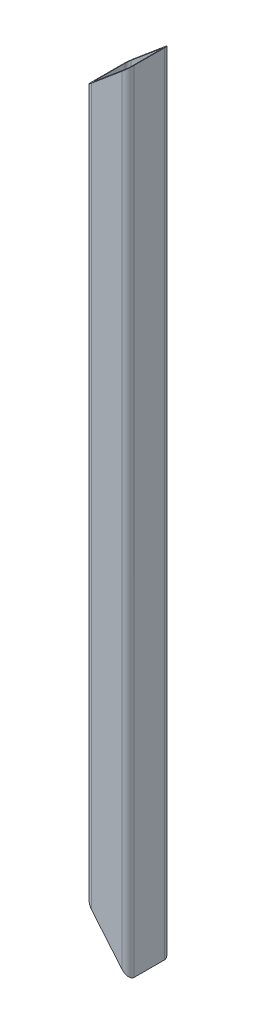
SolidWorks part; units mm, degrees
material "Q235B"
ref_plane "Front Plane" through (0, 0, 0) normal (0, 0, 1) x (1, 0, 0)
ref_plane "Top Plane" through (0, 0, 0) normal (0, 1, 0) x (1, 0, 0)
ref_plane "Right Plane" through (0, 0, 0) normal (1, 0, 0) x (0, 0, -1)
sketch "feature 17 (ProfileFeature) (+16 more in 12 files) Sketch1" plane through (0, 0, 0) normal (0, 0, 1) x (1, 0, 0)
  line L0 (0, 0) -> (0, 1302)
  dimension "D1" = 1302
other "feature 19 (WeldMemberFeat) (+4 more in 5 files) Cold-formed Hollow Structural Square Steel(gb t6728-2002) 70×70×5(1)"
ref_plane "Plane1" through (0, 0, 0) normal (0, 1, 0) x (-1, 0, 0)
sketch "Sketch1" plane through (0, 0, 0) normal (0, 1, 0) x (-1, 0, 0)
  line L0 (-25, -30) -> (25, -30)
  line L1 (-30, -25) -> (-30, 25)
  line L2 (25, 30) -> (-25, 30)
  line L3 (30, 25) -> (30, -25)
  line L4 (-25, -35) -> (25, -35)
  line L5 (-35, -25) -> (-35, 25)
  line L6 (25, 35) -> (-25, 35)
  line L7 (35, 25) -> (35, -25)
  arc A0 (35, 25) -> (25, 35) centre (25, 25) ccw
  arc A1 (25, -35) -> (35, -25) centre (25, -25) ccw
  arc A2 (-35, -25) -> (-25, -35) centre (-25, -25) ccw
  arc A3 (-25, 35) -> (-35, 25) centre (-25, 25) ccw
  arc A4 (-25, 30) -> (-30, 25) centre (-25, 25) ccw
  arc A5 (30, 25) -> (25, 30) centre (25, 25) ccw
  arc A6 (25, -30) -> (30, -25) centre (25, -25) ccw
  arc A7 (-30, -25) -> (-25, -30) centre (-25, -25) ccw
  point P0 (-35, 0)
  point P1 (35, 0)
  point P2 (0, 35)
  point P3 (0, -35)
  point P4 (0, 0)
  point P5 (-35, -35)
  point P6 (35, -35)
  point P7 (35, 35)
  point P8 (-35, 35)
  point P33 (0, 0)
  dimension "D1" = 10
  dimension "D2" = 70
  dimension "D3" = 5
sketch "0:feat:20/0 feature 20/0 (ProfileFeature) (+11 more in 7 files) Sketch2" plane through (0, 0, 35) normal (0, 0, 1) x (1, 0, 0)
  line L0 (35, 1302) -> (-35, 1243.247)
  line L1 (-35, 1302) -> (-35, 0) construction
  line L2 (-35, 1243.247) -> (-35, 1302)
  line L3 (-35, 1302) -> (35, 1302)
  line L4 (-35, 83.4) -> (35, 0)
  line L5 (35, 0) -> (-35, 0)
  line L6 (-35, 0) -> (-35, 83.4)
  dimension "D1" = 83.4
  dimension "D2" = 90
extrude "Cut-Extrude1" cut sketch "0:feat:20/0 feature 20/0 (ProfileFeature) (+11 more in 7 files) Sketch2" against normal through all both and the other way through all
